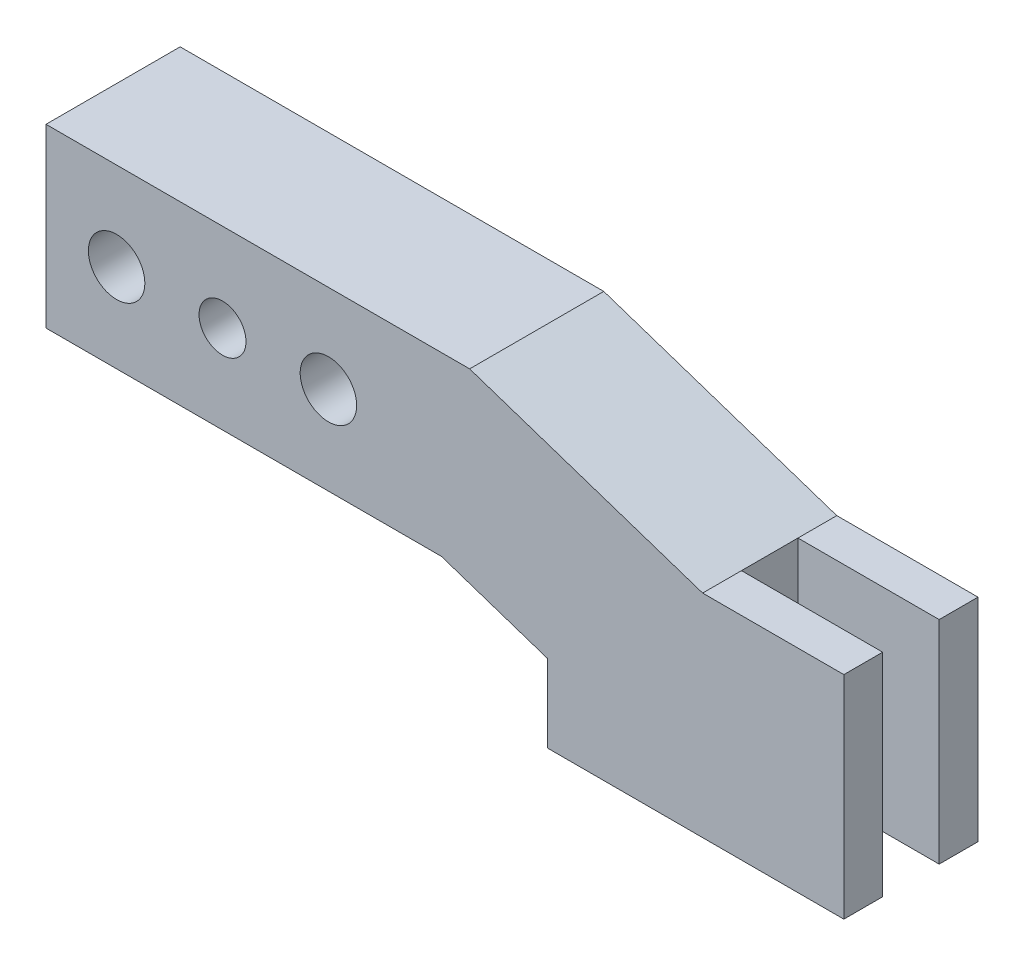
SolidWorks part; units mm, degrees
ref_plane "Front Plane" through (0, 0, 0) normal (0, 0, 1) x (1, 0, 0)
ref_plane "Top Plane" through (0, 0, 0) normal (0, 1, 0) x (1, 0, 0)
ref_plane "Right Plane" through (0, 0, 0) normal (1, 0, 0) x (0, 0, -1)
sketch "Sketch1" plane through (0, 0, 0) normal (0, 0, 1) x (1, 0, 0)
  line L0 (0, 0) -> (56, 0)
  line L1 (56, 0) -> (71, -5)
  line L2 (71, -5) -> (71, -16)
  line L3 (71, -16) -> (113, -16)
  line L4 (113, -16) -> (113, 14)
  line L5 (113, 14) -> (93, 14)
  line L6 (93, 14) -> (60, 25)
  line L7 (60, 25) -> (0, 25)
  line L8 (0, 25) -> (0, 0)
  line L9 (0, 12.5) -> (63.7299, 12.5) construction
  circle A0 centre (10, 12.5) radius 4
  circle A1 centre (25, 12.5) radius 3.3235
  circle A2 centre (40, 12.5) radius 4
  dimension "D10" = 10
  dimension "D11" = 15
  dimension "D12" = 15
  dimension "D1" = 25
  dimension "D2" = 56
  dimension "D3" = 60
  dimension "D4" = 20
  dimension "D5" = 42
  dimension "D6" = 30
  dimension "D7" = 11
  dimension "D8" = 5
  dimension "D9" = 15
extrude "Boss-Extrude1" add sketch "Sketch1" along normal blind 19
ref_plane "Plane1" through (0, 14, 0) normal (0, 1, 0) x (1, 0, 0)
sketch "Sketch2" plane through (0, 14, 0) normal (0, 1, 0) x (1, 0, 0)
  line L0 (93, -19) -> (93, 0) construction
  line L1 (93, -5.5) -> (113, -5.5)
  line L2 (93, -5.5) -> (93, -13.5)
  line L3 (93, -13.5) -> (113, -13.5)
  line L4 (113, -5.5) -> (113, -13.5)
  line L5 (113, -19) -> (113, 0) construction
  line L6 (113, -19) -> (93, -19) construction
  line L7 (113, 0) -> (93, 0) construction
  dimension "D1" = 5.5
  dimension "D2" = 5.5
extrude "Cut-Extrude1" cut sketch "Sketch2" against normal up to next
ref_plane "Plane2" through (0, -16, 0) normal (0, -1, 0) x (-1, 0, 0)
sketch "Sketch3" plane through (0, -16, 0) normal (0, -1, 0) x (-1, 0, 0)
  line L0 (-93, -9.5) -> (-71, -9.5) construction
  line L1 (-93, -13.5) -> (-93, -5.5) construction
  line L2 (-71, -19) -> (-71, 0) construction
  line L3 (-71, -19) -> (-71, 0) construction
  circle A0 centre (-79, -9.5) radius 2.4585
  dimension "D1" = 8
extrude "Cut-Extrude2" cut sketch "Sketch3" against normal blind 15
